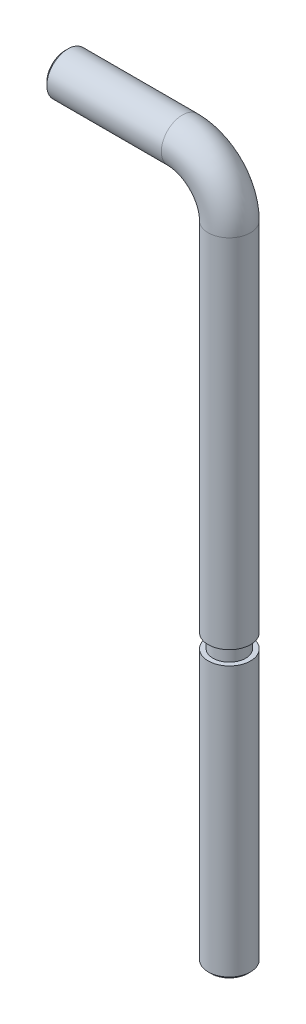
from build123d import *

# Parameters (mm, degrees)
SKETCH2_R     = 2.25
SKETCH3_W     = 0.5
SKETCH3_H     = 1.5
CHAMFER1_SIZE = 0.3


with BuildPart() as part:
    # Sweep1: sweep along a path in Sketch1
    with BuildLine(Plane.XY) as sweep1_path:
        Line((0, 0), (0, 68.5))
        ThreePointArc((0, 68.5), (-1.464466094, 72.035533906), (-5, 73.5))
        Line((-5, 73.5), (-17.5, 73.5))
    # Sketch2 → Sweep1 (sweep)
    with BuildSketch(Plane(origin=(0, 0, 0), x_dir=(1, 0, 0), z_dir=(0, 1, 0))):
        Circle(SKETCH2_R)
    sweep(path=sweep1_path.line)

    # Sketch3 → Cut-Revolve1 (revolve, cut)
    with BuildSketch(Plane(origin=(0, 0, 0), x_dir=(0, 0, -1), z_dir=(1, 0, 0))):
        with Locations((2, 29.75)):
            Rectangle(SKETCH3_W, SKETCH3_H)
    revolve(axis=Axis((0, 0, 0), (0, 1, 0)), mode=Mode.SUBTRACT)

    # Chamfer1
    chamfer1_edges = [part.edges().sort_by_distance(p)[0] for p in [
        (-2.25, 0, 0),
        (-17.5, 71.25, 0),
    ]]
    chamfer(chamfer1_edges, length=CHAMFER1_SIZE)


solid = part.part
